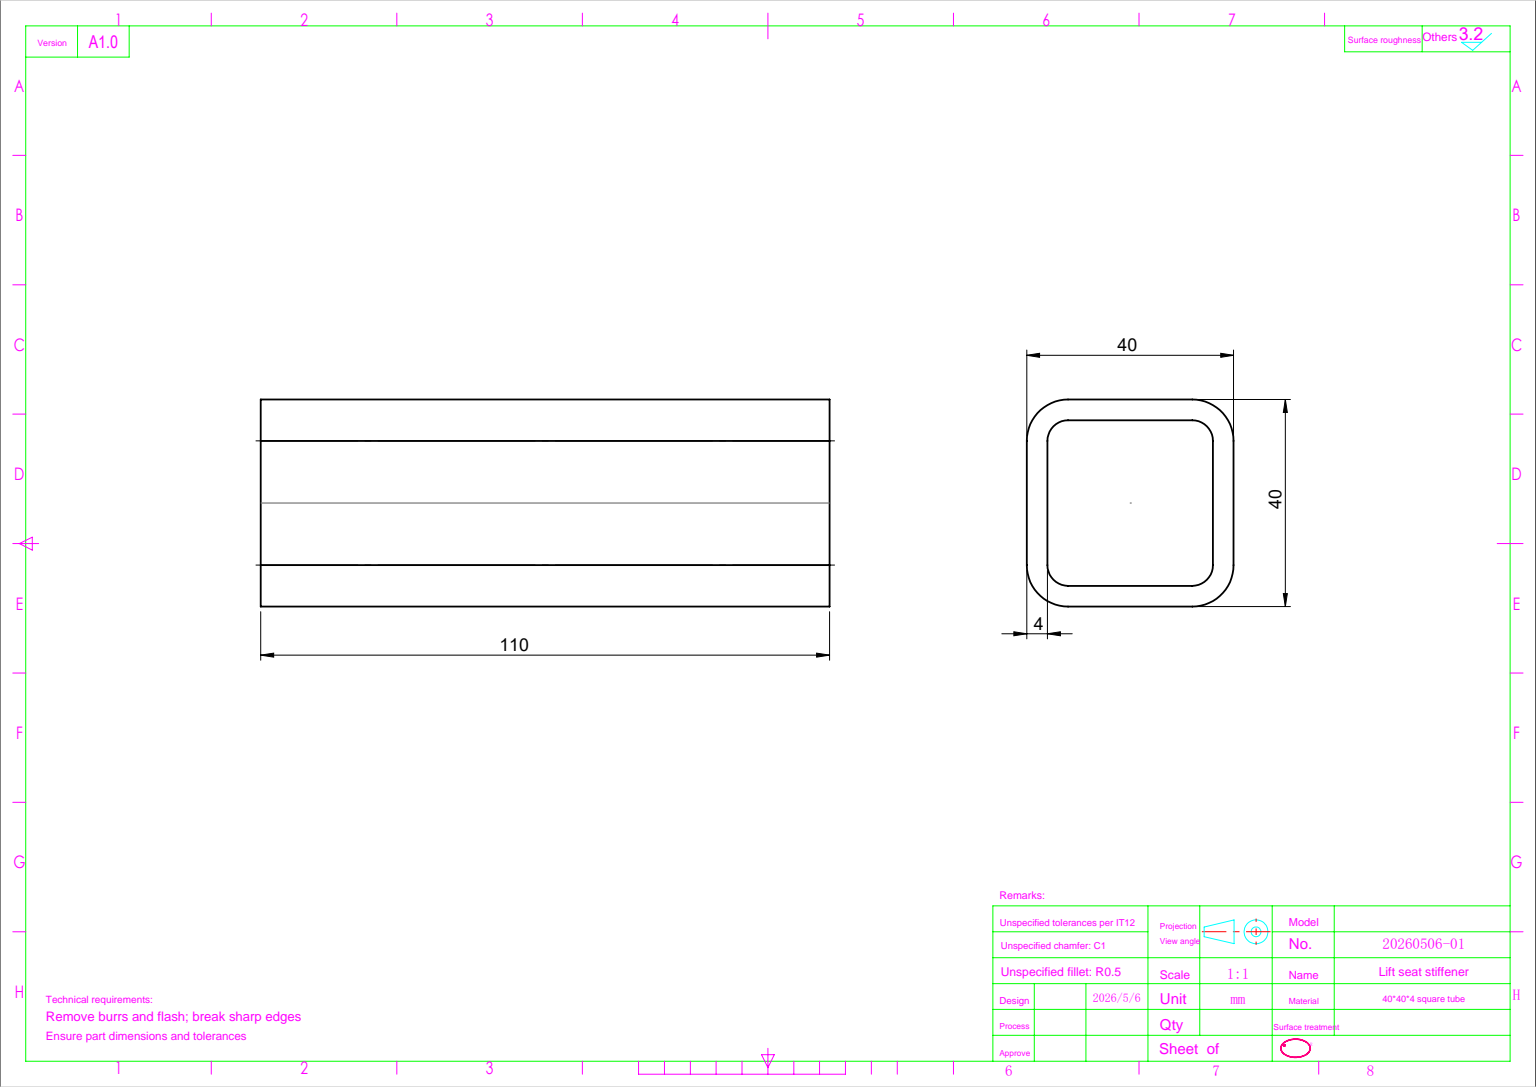
from build123d import *

# Parameters (mm, degrees)
F_40_X_40_X_4_1_DEPTH = 110


with BuildPart() as part:
    # Sketch12 → 方形管 40 X 40 X 4(1) (new body)
    with BuildSketch(Plane(origin=(0, 0, 0), x_dir=(0, 0, -1), z_dir=(1, 0, 0))):
        with BuildLine():
            Line((-12, -20), (12, -20))
            ThreePointArc((12, -20), (17.656854249, -17.656854249), (20, -12))
            Line((20, -12), (20, 12))
            ThreePointArc((20, 12), (17.656854249, 17.656854249), (12, 20))
            Line((12, 20), (-12, 20))
            ThreePointArc((-12, 20), (-17.656854249, 17.656854249), (-20, 12))
            Line((-20, 12), (-20, -12))
            ThreePointArc((-20, -12), (-17.656854249, -17.656854249), (-12, -20))
        make_face()
        with BuildLine():
            Line((-12, -16), (12, -16))
            ThreePointArc((12, -16), (14.828427125, -14.828427125), (16, -12))
            Line((16, -12), (16, 12))
            ThreePointArc((16, 12), (14.828427125, 14.828427125), (12, 16))
            Line((12, 16), (-12, 16))
            ThreePointArc((-12, 16), (-14.828427125, 14.828427125), (-16, 12))
            Line((-16, 12), (-16, -12))
            ThreePointArc((-16, -12), (-14.828427125, -14.828427125), (-12, -16))
        make_face(mode=Mode.SUBTRACT)
    extrude(amount=F_40_X_40_X_4_1_DEPTH)


solid = part.part
